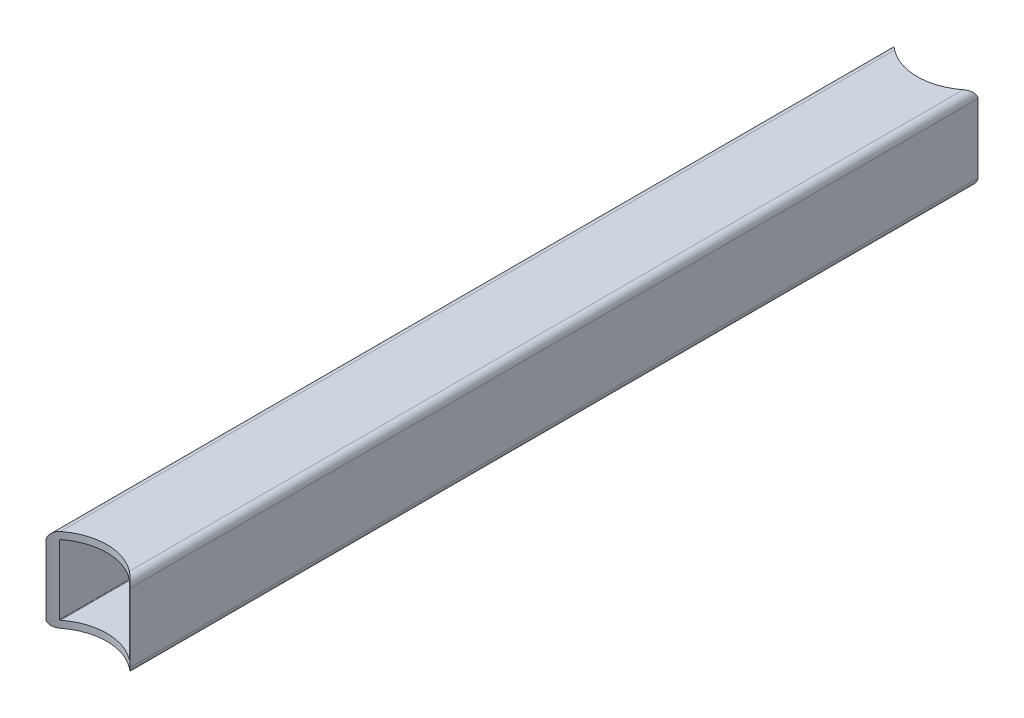
from build123d import *

# Parameters (mm, degrees)
EXTRUDE_1_DEPTH     = 165
SKETCH_3_R          = 20
CUT_EXTRUDE_1_DEPTH = 25


with BuildPart() as part:
    # 草图2 → 拉伸-薄壁1 (new, symmetric)
    with BuildSketch(Plane.XY):
        with BuildLine():
            Line((-12.3, 15), (12.3, 15))
            ThreePointArc((12.3, 15), (14.209188309, 14.209188309), (15, 12.3))
            Line((15, 12.3), (15, -12.3))
            ThreePointArc((15, -12.3), (14.209188309, -14.209188309), (12.3, -15))
            Line((12.3, -15), (-12.3, -15))
            ThreePointArc((-12.3, -15), (-14.209188309, -14.209188309), (-15, -12.3))
            Line((-15, -12.3), (-15, 12.3))
            ThreePointArc((-15, 12.3), (-14.209188309, 14.209188309), (-12.3, 15))
        make_face()
        with BuildLine():
            Line((-12.3, 12.5), (12.3, 12.5))
            ThreePointArc((12.3, 12.5), (12.441421356, 12.441421356), (12.5, 12.3))
            Line((12.5, 12.3), (12.5, -12.3))
            ThreePointArc((12.5, -12.3), (12.441421356, -12.441421356), (12.3, -12.5))
            Line((12.3, -12.5), (-12.3, -12.5))
            ThreePointArc((-12.3, -12.5), (-12.441421356, -12.441421356), (-12.5, -12.3))
            Line((-12.5, -12.3), (-12.5, 12.3))
            ThreePointArc((-12.5, 12.3), (-12.441421356, 12.441421356), (-12.3, 12.5))
        make_face(mode=Mode.SUBTRACT)
    extrude(amount=EXTRUDE_1_DEPTH, both=True)

    # 草图3 → 切除-拉伸1 (cut, symmetric)
    with BuildSketch(Plane(origin=(0, 0, 0), x_dir=(1, 0, 0), z_dir=(0, 1, 0))):
        with Locations((0, -165)):
            Circle(SKETCH_3_R)
        with Locations((0, 165)):
            Circle(SKETCH_3_R)
    extrude(amount=CUT_EXTRUDE_1_DEPTH, both=True, mode=Mode.SUBTRACT)


solid = part.part
